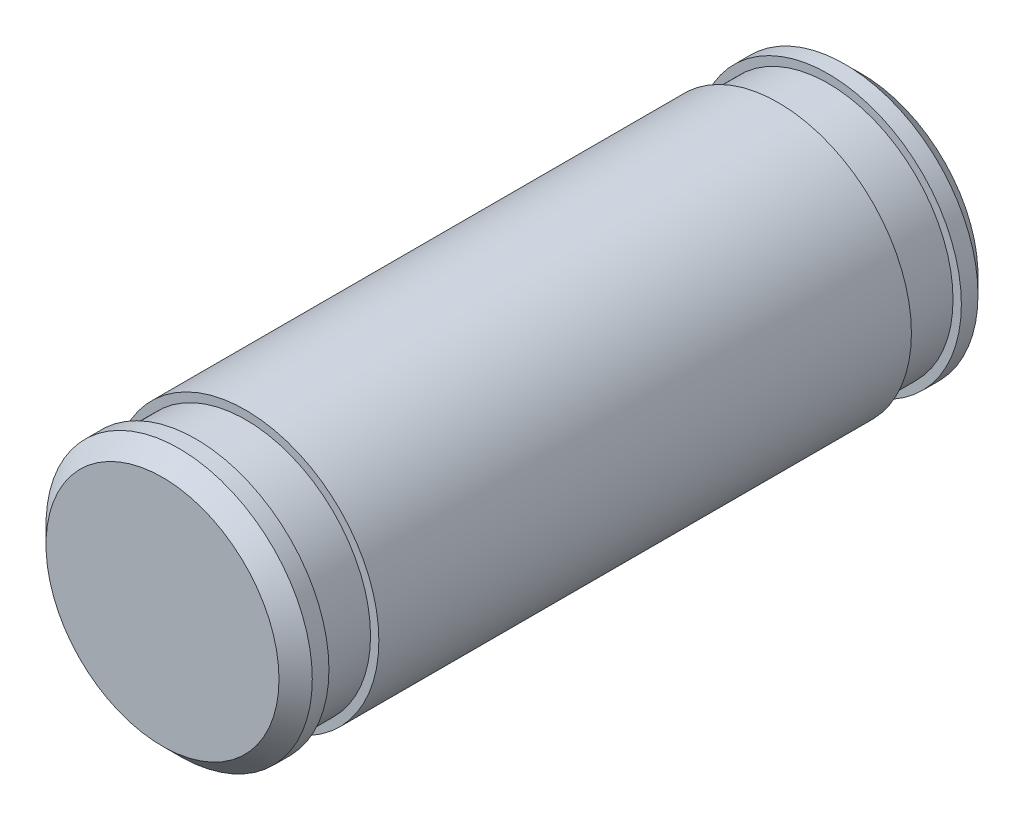
SolidWorks part; units mm, degrees
ref_plane "Front Plane" through (0, 0, 0) normal (0, 0, 1) x (1, 0, 0)
ref_plane "Top Plane" through (0, 0, 0) normal (0, 1, 0) x (1, 0, 0)
ref_plane "Right Plane" through (0, 0, 0) normal (1, 0, 0) x (0, 0, -1)
other "Configuration Table"
sketch "Sketch1" plane through (0, 0, 0) normal (0, 0, 1) x (1, 0, 0)
  circle A0 centre (0, 0) radius 4
  dimension "D1" = 8
extrude "Boss-Extrude1" add sketch "Sketch1" along normal mid plane 16
sketch "Sketch2" plane through (0, 0, 8) normal (0, 0, 1) x (1, 0, 0)
  circle A0 centre (0, 0) radius 3.75
  dimension "D1" = 7.5
extrude "Boss-Extrude2" add sketch "Sketch2" along normal blind 1.5
sketch "Sketch3" plane through (0, 0, 9.5) normal (0, 0, 1) x (1, 0, 0)
  circle A0 centre (0, 0) radius 4
  dimension "D1" = 8
extrude "Boss-Extrude3" add sketch "Sketch3" along normal blind 1
chamfer "Chamfer1" distance 0.5 angle 45 1 edges at (4, 0, 10.5)
mirror "Mirror1" about plane through (0, 0, 0) normal (0, 0, 1) of "Boss-Extrude2", "Boss-Extrude3", "Chamfer1"
